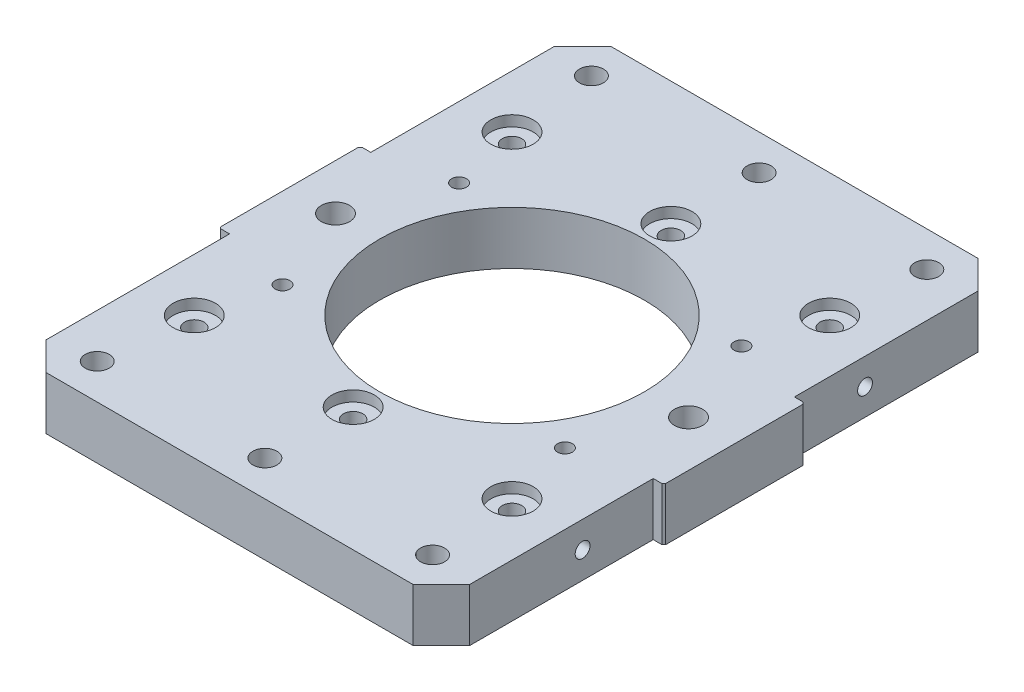
SolidWorks part; units mm, degrees
ref_plane "Front Plane" through (0, 0, 0) normal (0, 0, 1) x (1, 0, 0)
ref_plane "Top Plane" through (0, 0, 0) normal (0, 1, 0) x (1, 0, 0)
ref_plane "Right Plane" through (0, 0, 0) normal (1, 0, 0) x (0, 0, -1)
sketch "Sketch1" plane through (0, 0, 0) normal (0, 1, 0) x (1, 0, 0)
  line L1 (-60, 80) -> (60, 80)
  line L2 (-60, 80) -> (-60, -80)
  line L3 (-60, -80) -> (60, -80)
  line L4 (60, 80) -> (60, -80)
  line L5 (-60, 80) -> (60, -80) construction
  line L6 (-60, -80) -> (60, 80) construction
  point P0 (0, 0)
  dimension "D1" = 120
  dimension "D2" = 160
extrude "Boss-Extrude1" add sketch "Sketch1" along normal blind 15
chamfer "Chamfer1" distance 8 angle 45 4 edges at (-60, 7.5, -80) (-60, 7.5, 80) (60, 7.5, -80) (60, 7.5, 80)
sketch "Sketch2" plane through (0, 15, 0) normal (0, 1, 0) x (1, 0, 0)
  circle A0 centre (0, 0) radius 37.5
  dimension "D1" = 75
extrude "Cut-Extrude1" cut sketch "Sketch2" against normal blind 23
sketch "Sketch3" plane through (0, 0, 0) normal (0, -1, 0) x (1, 0, 0)
  line L0 (0, 0) -> (50000, 0) construction
  line L1 (0, 0) -> (0, -50000) construction
  circle A0 centre (-40, 25) radius 1
  circle A1 centre (40, 25) radius 1
  circle A2 centre (-40, -25) radius 1
  circle A3 centre (40, -25) radius 1
  dimension "D2" = 80
  dimension "D3" = 2
  dimension "D1" = 50
extrude "Cut-Extrude2" cut sketch "Sketch3" against normal blind 10
hole_wizard "M5 Tapped Hole1" positions "3DSketch2" profile "Sketch7" tap size "M5" standard "Gb" end condition through all
sketch3d "3DSketch2"
  line L0 (-40, 10, 25) -> (-40, 0, 25) construction
  line L1 (40, 10, 25) -> (40, 0, 25) construction
  line L2 (40, 10, -25) -> (40, 0, -25) construction
  line L3 (-40, 10, -25) -> (-40, 0, -25) construction
  point P0 (-40, 0, 25)
  point P4 (40, 0, 25)
  point P8 (40, 0, -25)
  point P12 (-40, 0, -25)
sketch "Sketch7" plane through (-40, 0, 25) normal (1, 0, 0) x (0, 0, -1)
  line L0 (0, 0) -> (0, 15)
  line L1 (0, 15) -> (2.1, 15)
  line L2 (2.1, 15) -> (2.1, 0)
  line L5 (2.1, 0) -> (0, 0)
  line L11 (0, -6.35) -> (0, 107.95) construction
  dimension "通孔螺纹孔钻头直径" = 4.2
  dimension "通孔螺纹孔钻头深度" = 15
cosmetic thread "Cosmetic Thread1" parameters "D2"=5
cosmetic thread "Cosmetic Thread2" parameters "D2"=5
cosmetic thread "Cosmetic Thread3" parameters "D2"=5
cosmetic thread "Cosmetic Thread4" parameters "D2"=5
sketch "Sketch8" plane through (0, 0, 0) normal (0, -1, 0) x (1, 0, 0)
  line L0 (0, 75) -> (0, -49925) construction
  line L1 (-52, 80) -> (52, 80) construction
  line L2 (0, 0) -> (50000, 0) construction
  line L3 (-45.8917, 70) -> (49954.1083, 70) construction
  circle A0 centre (-47.5, 70) radius 3
  circle A1 centre (0, 70) radius 3
  circle A2 centre (47.5, 70) radius 3
  circle A3 centre (47.5, -70) radius 3
  circle A4 centre (0, -70) radius 3
  circle A5 centre (-47.5, -70) radius 3
  point P4 (0, 80)
  dimension "D1" = 6
  dimension "D2" = 95
  dimension "D3" = 140
extrude "Cut-Extrude4" cut sketch "Sketch8" against normal blind 55
hole_wizard "M8 Tapped Hole1" positions "3DSketch3" profile "Sketch9" tap size "M8" standard "Gb" end condition through all
sketch3d "3DSketch3"
  line L0 (47.5, 15, -70) -> (47.5, 0, -70) construction
  line L1 (0, 15, -70) -> (0, 0, -70) construction
  line L2 (-47.5, 15, -70) -> (-47.5, 0, -70) construction
  line L3 (-47.5, 15, 70) -> (-47.5, 0, 70) construction
  line L4 (0, 15, 70) -> (0, 0, 70) construction
  line L5 (47.5, 15, 70) -> (47.5, 0, 70) construction
  point P0 (47.5, 0, -70)
  point P4 (0, 0, -70)
  point P8 (-47.5, 0, -70)
  point P12 (-47.5, 0, 70)
  point P16 (0, 0, 70)
  point P20 (47.5, 0, 70)
cosmetic thread "Cosmetic Thread5" parameters "D2"=8
cosmetic thread "Cosmetic Thread6" parameters "D2"=8
cosmetic thread "Cosmetic Thread7" parameters "D2"=8
cosmetic thread "Cosmetic Thread8" parameters "D2"=8
cosmetic thread "Cosmetic Thread9" parameters "D2"=8
cosmetic thread "Cosmetic Thread10" parameters "D2"=8
sketch "Sketch9" plane through (47.5, 0, -70) normal (1, 0, 0) x (0, 0, -1)
  line L0 (0, 0) -> (0, 15)
  line L1 (0, 15) -> (3.4, 15)
  line L2 (3.4, 15) -> (3.4, 0)
  line L5 (3.4, 0) -> (0, 0)
  line L11 (0, -6.35) -> (0, 107.95) construction
  dimension "通孔螺纹孔钻头直径" = 6.8
  dimension "通孔螺纹孔钻头深度" = 15
sketch "Sketch11" plane through (0, 0, 0) normal (0, -1, 0) x (1, 0, 0)
  line L0 (0, 0) -> (50000, 0) construction
  line L1 (0, 0) -> (0, 50000) construction
  circle A0 centre (-50, 0) radius 2.5
  circle A1 centre (50, 0) radius 2.5
  dimension "D1" = 5
  dimension "D2" = 100
extrude "Cut-Extrude5" cut sketch "Sketch11" against normal blind 33
sketch "Sketch12" plane through (0, 15, 0) normal (0, 1, 0) x (1, 0, 0)
  circle A0 centre (-50, 0) radius 4
  circle A1 centre (50, 0) radius 4
  dimension "D1" = 8
extrude "Cut-Extrude6" cut sketch "Sketch12" against normal blind 6
sketch "Sketch13" plane through (0, 15, 0) normal (0, 1, 0) x (1, 0, 0)
  line L0 (0, 0) -> (0, 50000) construction
  line L1 (0, 0) -> (50000, 0) construction
  line L2 (-60, 72) -> (-60, -72) construction
  line L3 (-63, 20) -> (-60, 20)
  line L4 (-63, 20) -> (-63, -20)
  line L5 (-63, -20) -> (-60, -20)
  line L6 (-60, 20) -> (-60, -20)
  line L7 (-63, 20) -> (-60, -20) construction
  line L8 (-63, -20) -> (-60, 20) construction
  line L9 (63, -20) -> (60, 20) construction
  line L10 (63, 20) -> (60, -20) construction
  line L11 (60, 20) -> (60, -20)
  line L12 (63, -20) -> (60, -20)
  line L13 (63, 20) -> (63, -20)
  line L14 (63, 20) -> (60, 20)
  point P5 (-61.5, 0)
  point P16 (61.5, 0)
  dimension "D1" = 40
  dimension "D2" = 3
extrude "Boss-Extrude2" add sketch "Sketch13" against normal up to surface (15 mm away) up to face at (50, 0, 2.5)
chamfer "Chamfer2" distance 0.5 angle 45 4 edges at (63, 7.5, -20) (63, 7.5, 20) (-63, 7.5, -20) (-63, 7.5, 20)
sketch "Sketch14" plane through (60, 0, 0) normal (1, 0, 0) x (0, 0, -1)
  circle A0 centre (-40, 7.5) radius 1.7942
  circle A1 centre (40, 7.5) radius 1.7564
extrude "Cut-Extrude7" cut sketch "Sketch14" against normal blind 5
hole_wizard "M5 Tapped Hole2" positions "3DSketch4" profile "Sketch15" tap size "M5" standard "Gb"
sketch3d "3DSketch4"
  line L0 (55, 7.5, 40) -> (60, 7.5, 40) construction
  line L1 (55, 7.5, -40) -> (60, 7.5, -40) construction
  point P0 (60, 7.5, 40)
  point P8 (60, 7.5, -40)
sketch "Sketch15" plane through (60, 7.5, 40) normal (0, 1, 0) x (0, 0, -1)
  line L0 (0, 0) -> (0, 13.6618)
  line L1 (0, 13.6618) -> (2.1, 12.4)
  line L2 (2.1, 12.4) -> (2.1, 0)
  line L5 (2.1, 0) -> (0, 0)
  line L10 (0, 13.6618) -> (-2.1, 12.4) construction
  line L11 (0, -6.35) -> (0, 107.95) construction
  dimension "螺纹孔钻头直径" = 4.2
  dimension "螺纹孔钻头深度" = 12.4
  dimension "导头角度" = 118
cosmetic thread "Cosmetic Thread11" parameters "D1"=10, "D2"=5
cosmetic thread "Cosmetic Thread12" parameters "D1"=10, "D2"=5
mirror "Mirror1" about plane through (0, 0, 0) normal (1, 0, 0) of "M5 Tapped Hole2"
sketch "Sketch16" plane through (0, 15, 0) normal (0, 1, 0) x (1, 0, 0)
  line L0 (-37.5, 0) -> (49962.5, 0) construction
  line L1 (0, 37.5) -> (0, -49962.5) construction
  circle A2 centre (0, 45) radius 2.75
  circle A3 centre (45, 45) radius 2.75
  circle A4 centre (-45, 45) radius 2.75
  circle A5 centre (-45, -45) radius 2.75
  circle A6 centre (45, -45) radius 2.75
  circle A7 centre (0, -45) radius 2.75
  dimension "D2" = 90
  dimension "D3" = 5.5
  dimension "D1" = 90
extrude "Cut-Extrude8" cut sketch "Sketch16" against normal blind 55
sketch "Sketch17" plane through (0, 15, 0) normal (0, 1, 0) x (1, 0, 0)
  circle A0 centre (-45, -45) radius 6
  circle A1 centre (0, -45) radius 6
  circle A2 centre (45, -45) radius 6
  circle A3 centre (0, 45) radius 6
  circle A4 centre (45, 45) radius 6
  circle A5 centre (-45, 45) radius 6
  dimension "D1" = 12
extrude "Cut-Extrude9" cut sketch "Sketch17" against normal blind 3
